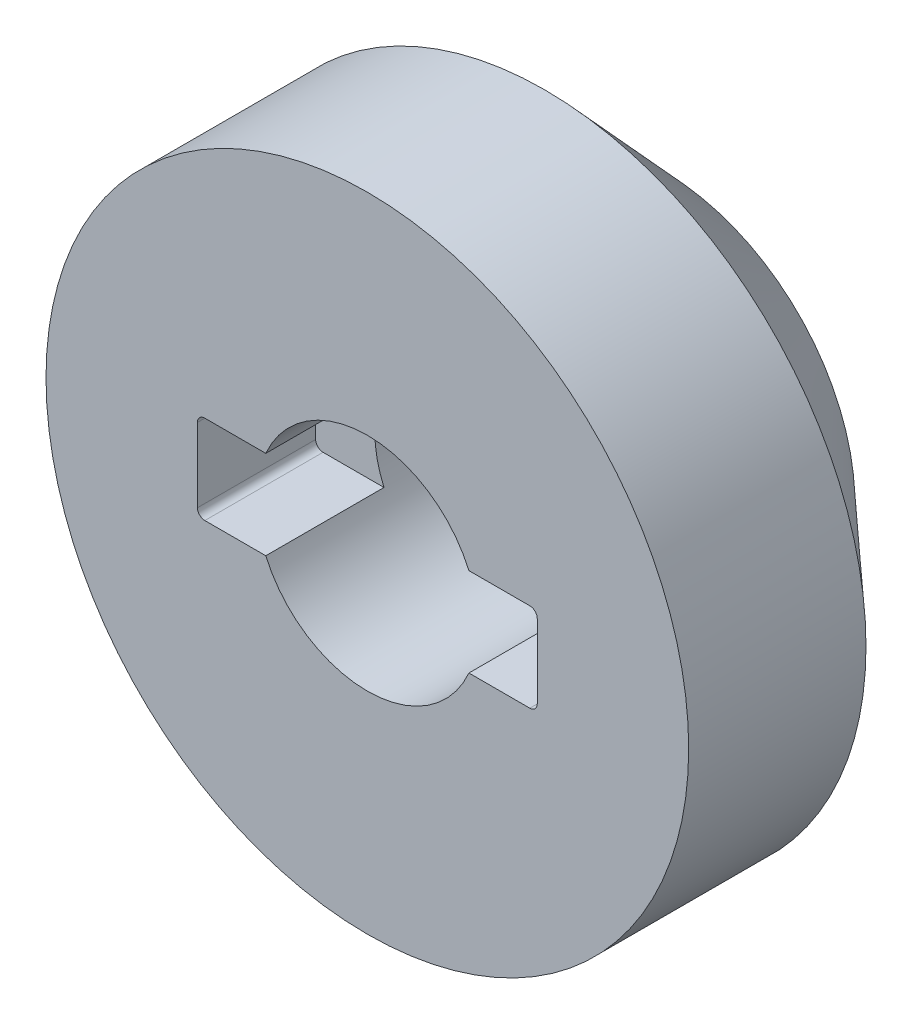
from build123d import *

# Parameters (mm, degrees)
SKETCH_1_R          = 21.75
SKETCH_1_R_2        = 7.5
EXTRUDE_1_DEPTH     = 12
CUT_EXTRUDE_1_DEPTH = 8
SKETCH_4_R          = 21.75
SKETCH_5_R          = 13
SKETCH_6_R          = 6.5
CUT_EXTRUDE_3_DEPTH = 48


with BuildPart() as part:
    # 草图1 → 凸台-拉伸1 (new body)
    with BuildSketch(Plane.XY):
        Circle(SKETCH_1_R)
        Circle(SKETCH_1_R_2, mode=Mode.SUBTRACT)
    extrude(amount=EXTRUDE_1_DEPTH)

    # 草图2 → 切除-拉伸1 (cut)
    with BuildSketch(Plane.XY.offset(12)):
        with BuildLine():
            Line((-11, 3), (11, 3))
            ThreePointArc((11, 3), (11.353553391, 2.853553391), (11.5, 2.5))
            Line((11.5, 2.5), (11.5, -2.5))
            ThreePointArc((11.5, -2.5), (11.353553391, -2.853553391), (11, -3))
            Line((11, -3), (-11, -3))
            ThreePointArc((-11, -3), (-11.353553391, -2.853553391), (-11.5, -2.5))
            Line((-11.5, -2.5), (-11.5, 2.5))
            ThreePointArc((-11.5, 2.5), (-11.353553391, 2.853553391), (-11, 3))
        make_face()
    extrude(amount=-CUT_EXTRUDE_1_DEPTH, mode=Mode.SUBTRACT)

    # 草图4 → 放样2 section 0
    with BuildSketch(Plane(origin=(0, 0, 0), x_dir=(-1, 0, 0), z_dir=(0, 0, -1))):
        Circle(SKETCH_4_R)
    # 草图5 → 放样2 section 1
    with BuildSketch(Plane(origin=(0, 0, -8), x_dir=(-1, 0, 0), z_dir=(0, 0, -1))):
        Circle(SKETCH_5_R)
    loft()

    # 草图6 → 切除-拉伸3 (cut)
    with BuildSketch(Plane.XY):
        Circle(SKETCH_6_R)
    extrude(amount=-CUT_EXTRUDE_3_DEPTH, mode=Mode.SUBTRACT)


solid = part.part
